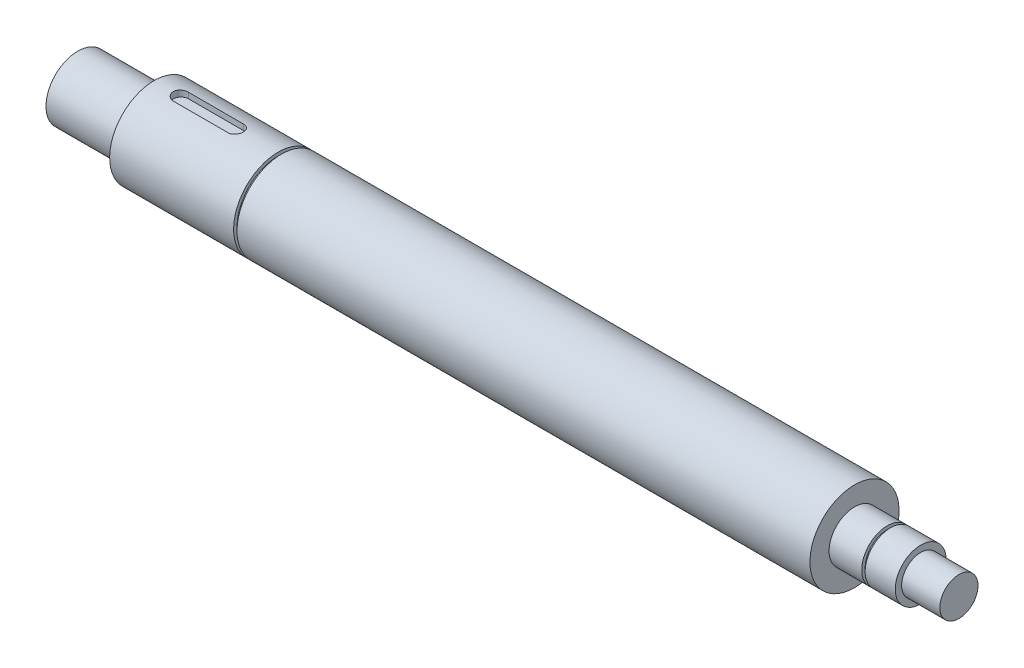
SolidWorks part; units mm, degrees
ref_plane "Front Plane" through (0, 0, 0) normal (0, 0, 1) x (1, 0, 0)
ref_plane "Top Plane" through (0, 0, 0) normal (0, 1, 0) x (1, 0, 0)
ref_plane "Right Plane" through (0, 0, 0) normal (1, 0, 0) x (0, 0, -1)
other "Configuration Table"
sketch "Sketch1" plane through (0, 0, 0) normal (0, 0, 1) x (1, 0, 0)
  line L0 (0, 0) -> (0, 25)
  line L1 (0, 25) -> (60, 25)
  line L2 (0, 0) -> (691.99, 0) construction
  line L3 (0, 0) -> (691.99, 0)
  line L4 (60, 25) -> (60, 35)
  line L5 (60, 35) -> (157.35, 35)
  line L10 (157.35, 35) -> (157.35, 32.35)
  line L11 (157.35, 32.35) -> (160, 32.35)
  line L12 (160, 32.35) -> (160, 35)
  line L13 (160, 35) -> (610, 35)
  line L14 (610, 35) -> (610, 20)
  line L15 (610, 20) -> (635.67, 20)
  line L16 (635.67, 20) -> (635.67, 17.35)
  line L17 (635.67, 17.35) -> (638.32, 17.35)
  line L18 (638.32, 17.35) -> (638.32, 20)
  line L19 (638.32, 20) -> (661.99, 20)
  line L20 (661.99, 20) -> (661.99, 15)
  line L21 (661.99, 15) -> (691.99, 15)
  line L22 (691.99, 15) -> (691.99, 0)
  dimension "D1" = 25
  dimension "D2" = 60
  dimension "D3" = 97.35
  dimension "D4" = 2.65
  dimension "D5" = 10
  dimension "D6" = 2.65
  dimension "D7" = 450
  dimension "D8" = 15
  dimension "D9" = 25.67
  dimension "D10" = 2.65
  dimension "D11" = 2.65
  dimension "D12" = 23.67
  dimension "D13" = 5
  dimension "D14" = 30
  dimension "D15" = 15
revolve "Revolve1" add sketch "Sketch1" angle 360 about L2
cosmetic thread "Cosmetic Thread1" parameters "D2"=49
cosmetic thread "Cosmetic Thread2" parameters "D2"=29
sketch "Sketch2" plane through (0, 0, 0) normal (0, 1, 0) x (1, 0, 0)
  line L0 (81, 0) -> (124, 0) construction
  line L1 (81, 6) -> (124, 6)
  line L2 (81, -6) -> (124, -6)
  line L6 (60, 35) -> (60, -35) construction
  arc A0 (81, 6) -> (81, -6) centre (81, 0) ccw
  arc A1 (124, -6) -> (124, 6) centre (124, 0) ccw
  point P3 (102.5, 0)
  dimension "D1" = 43
  dimension "D2" = 21
  dimension "D3" = 12
extrude "Cut-Extrude1" cut sketch "Sketch2" against normal blind 35 and the other way blind 1 from offset 65
